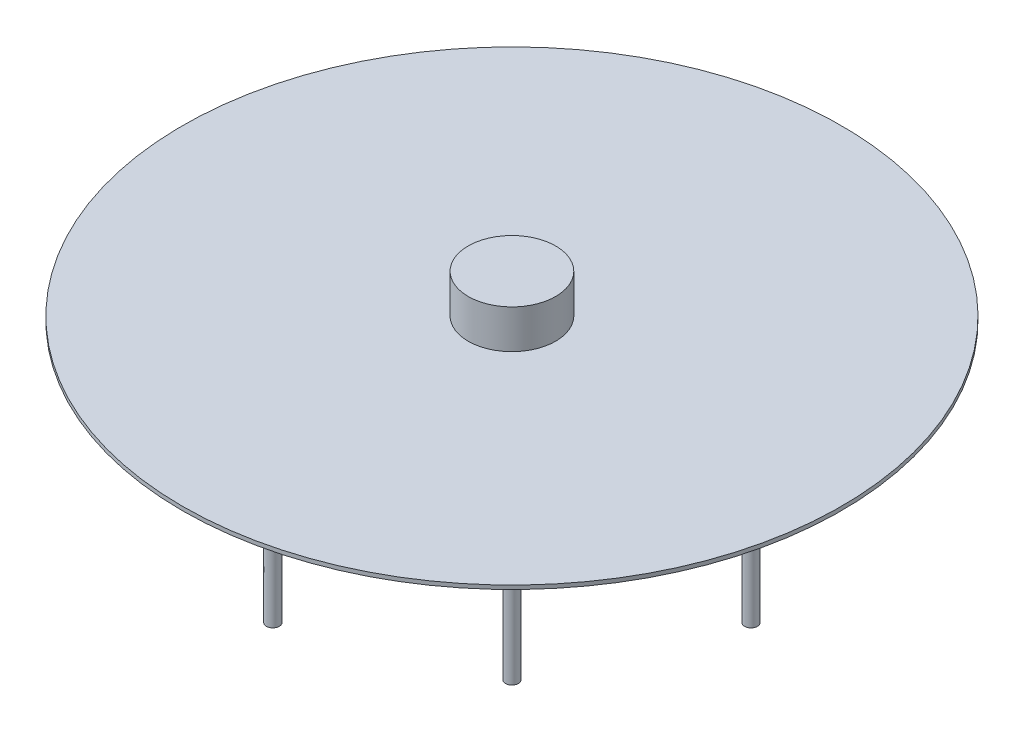
SolidWorks part; units mm, degrees
material "Power supply circuit board"
ref_plane "Front Plane" through (0, 0, 0) normal (0, 0, 1) x (1, 0, 0)
ref_plane "Top Plane" through (0, 0, 0) normal (0, 1, 0) x (1, 0, 0)
ref_plane "Right Plane" through (0, 0, 0) normal (1, 0, 0) x (0, 0, -1)
other "Configuration Table"
sketch "Sketch1" plane through (0, 0, 0) normal (0, 1, 0) x (1, 0, 0)
  circle A0 centre (0, 0) radius 225
  dimension "D1" = 450
extrude "Boss-Extrude2" add sketch "Sketch1" along normal blind 10 contours A0
sketch "Sketch2" plane through (0, 0, 0) normal (0, -1, 0) x (1, 0, 0)
  circle A0 centre (-185, 0) radius 5
  circle A1 centre (-130.8148, 130.8148) radius 5
  circle A2 centre (0, 185) radius 5
  circle A3 centre (130.8148, 130.8148) radius 5
  circle A4 centre (185, 0) radius 5
  circle A5 centre (130.8148, -130.8148) radius 5
  circle A6 centre (0, -185) radius 5
  circle A7 centre (-130.8148, -130.8148) radius 5
  point P19 (0, 0)
  dimension "D1" = 185
  dimension "D2" = 8
extrude "Boss-Extrude3" add sketch "Sketch2" along normal blind 100
sketch "Sketch3" plane through (0, 10, 0) normal (0, 1, 0) x (1, 0, 0)
  circle A2 centre (0, 0) radius 255
  circle A3 centre (0, 0) radius 255
  dimension "D1" = 30
extrude "Boss-Extrude5" add sketch "Sketch3" along normal blind 3
sketch "Sketch7" plane through (0, 13, 0) normal (0, 1, 0) x (1, 0, 0)
  circle A0 centre (0, 0) radius 33.8495
extrude "Boss-Extrude6" add sketch "Sketch7" along normal blind 30
